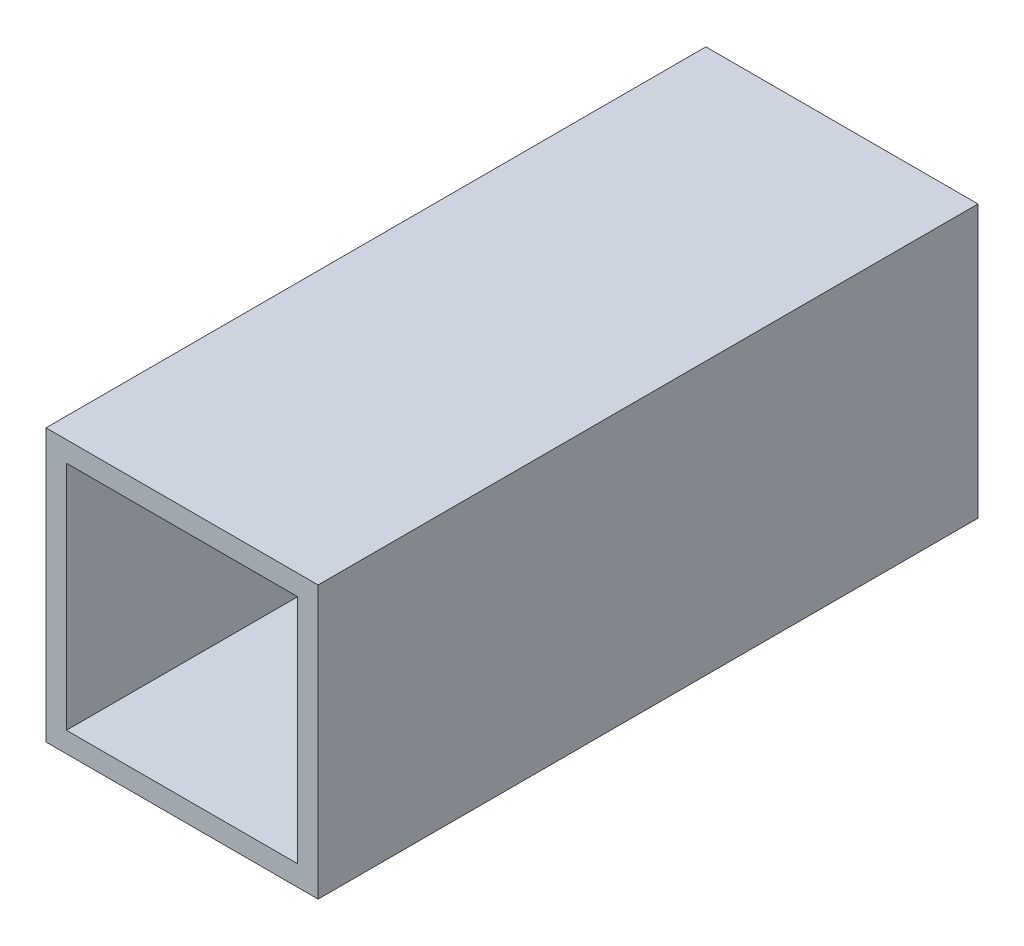
SolidWorks part; units mm, degrees
ref_plane "前视基准面" through (0, 0, 0) normal (0, 0, 1) x (1, 0, 0)
ref_plane "上视基准面" through (0, 0, 0) normal (0, 1, 0) x (1, 0, 0)
ref_plane "右视基准面" through (0, 0, 0) normal (1, 0, 0) x (0, 0, -1)
other "Configuration Table"
sketch "草图1" plane through (0, 0, 0) normal (0, 0, 1) x (1, 0, 0)
  line L0 (-20, -20) -> (20, -20)
  line L1 (20, -20) -> (20, 20)
  line L2 (20, 20) -> (-20, 20)
  line L3 (-20, 20) -> (-20, -20)
  line L4 (-17, -17) -> (17, -17)
  line L5 (17, -17) -> (17, 17)
  line L6 (17, 17) -> (-17, 17)
  line L7 (-17, 17) -> (-17, -17)
  point P0 (0, 0)
  dimension "D1" = 3
  dimension "D2" = 20
  dimension "D3" = 37
  dimension "D4" = 40
  dimension "D5" = 3
  dimension "D6" = 20
  dimension "D7" = 37
  dimension "D8" = 40
extrude "凸台-拉伸1" add sketch "草图1" against normal mid plane 97
